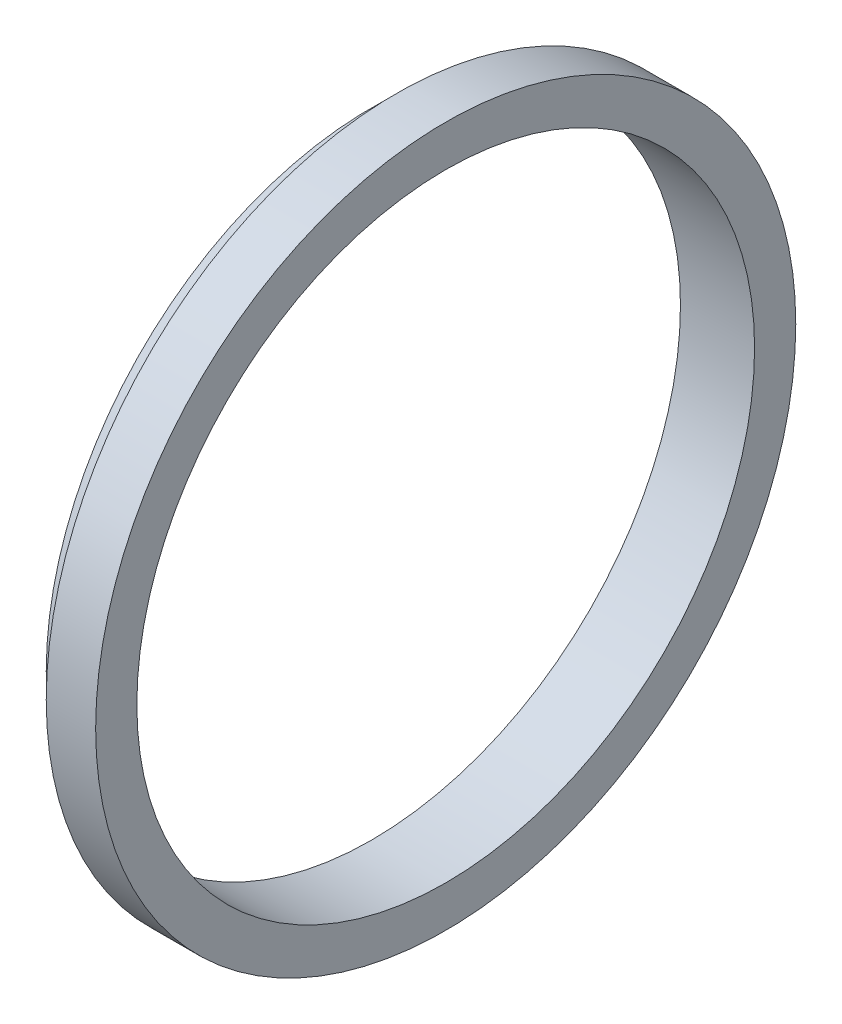
SolidWorks part; units mm, degrees
ref_plane "前视基准面" through (0, 0, 0) normal (0, 0, 1) x (1, 0, 0)
ref_plane "上视基准面" through (0, 0, 0) normal (0, 1, 0) x (1, 0, 0)
ref_plane "右视基准面" through (0, 0, 0) normal (1, 0, 0) x (0, 0, -1)
sketch "草图1" plane through (0, 0, 0) normal (0, 0, 1) x (1, 0, 0)
  line L0 (-9.1143, 0) -> (21.9882, 0) construction
  line L1 (0, 37.5) -> (9, 37.5)
  line L2 (9, 37.5) -> (9, 42.5)
  line L3 (9, 42.5) -> (3, 42.5)
  line L4 (0, 37.5) -> (0, 39.5)
  line L5 (3, 42.5) -> (3, 40.5)
  line L6 (0, 39.5) -> (3, 40.5)
  dimension "D1" = 9
  dimension "D2" = 5
  dimension "D3" = 6
  dimension "D4" = 2
  dimension "D5" = 2
  dimension "D6" = 37.5
revolve "旋转1" add sketch "草图1" angle 360 about L0
